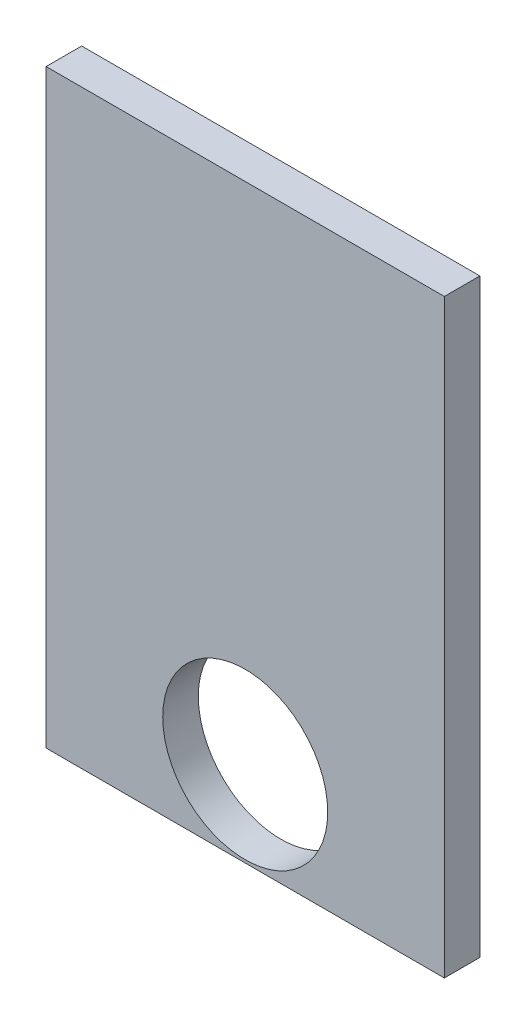
from build123d import *

# Parameters (mm, degrees)
SKETCH1_W           = 280
SKETCH1_H           = 415
SKETCH1_R           = 58
BOSS_EXTRUDE1_DEPTH = 25


with BuildPart() as part:
    # Sketch1 → Boss-Extrude1 (new body)
    with BuildSketch(Plane.XY):
        with Locations((140, -207.5)):
            Rectangle(SKETCH1_W, SKETCH1_H)
        with Locations((140, -355)):
            Circle(SKETCH1_R, mode=Mode.SUBTRACT)
    extrude(amount=BOSS_EXTRUDE1_DEPTH)


solid = part.part
